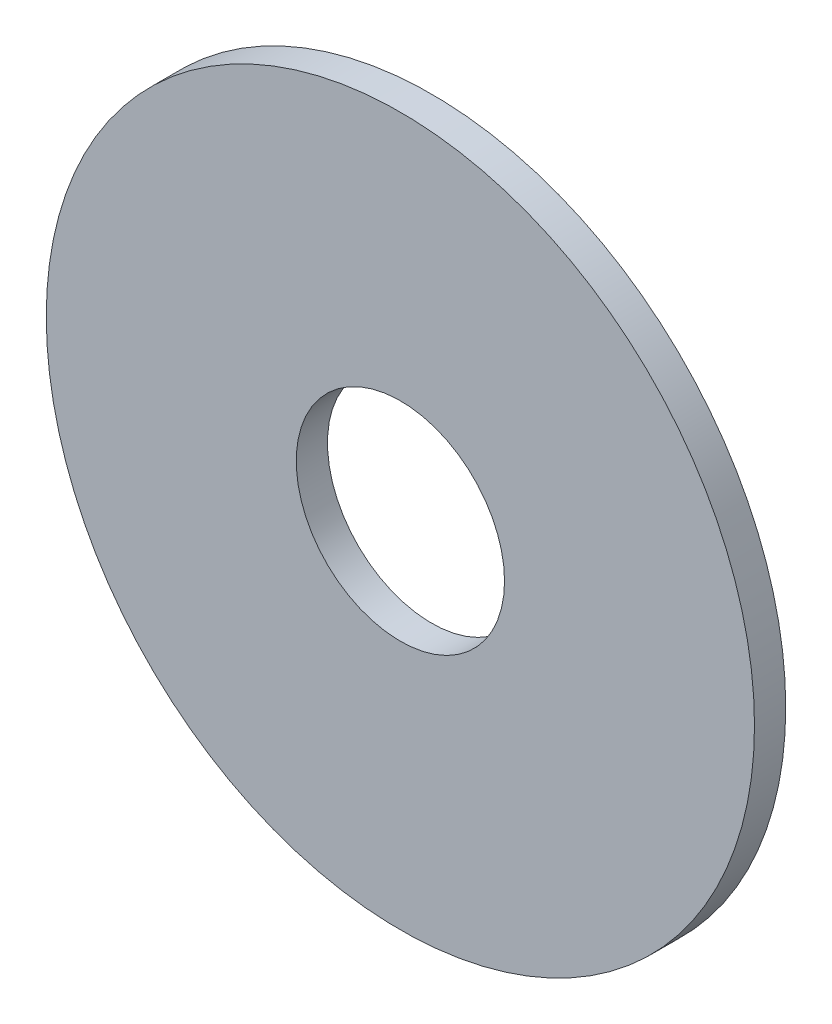
SolidWorks part; units mm, degrees
ref_plane "Front Plane" through (0, 0, 0) normal (0, 0, 1) x (1, 0, 0)
ref_plane "Top Plane" through (0, 0, 0) normal (0, 1, 0) x (1, 0, 0)
ref_plane "Right Plane" through (0, 0, 0) normal (1, 0, 0) x (0, 0, -1)
other "Configuration Table"
sketch "Sketch1" plane through (0, 0, 0) normal (0, 0, 1) x (1, 0, 0)
  circle A0 centre (0, 0) radius 85
  dimension "D1" = 170
extrude "Boss-Extrude1" add sketch "Sketch1" along normal blind 7.5
sketch "Sketch2" plane through (0, 0, 7.5) normal (0, 0, 1) x (1, 0, 0)
  circle A0 centre (0, 0) radius 25
  dimension "D1" = 50
extrude "Cut-Extrude1" cut sketch "Sketch2" against normal through all both and the other way through all
